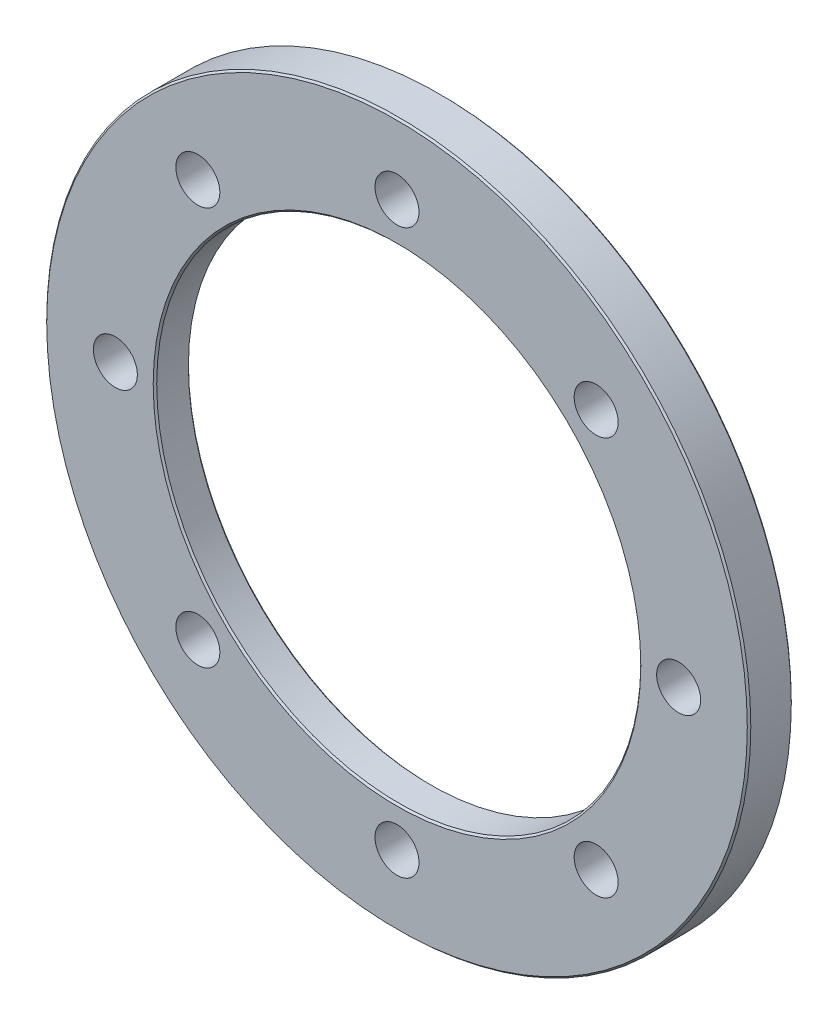
SolidWorks part; units mm, degrees
material "42CrMo"
ref_plane "Front Plane" through (0, 0, 0) normal (0, 0, 1) x (1, 0, 0)
ref_plane "Top Plane" through (0, 0, 0) normal (0, 1, 0) x (1, 0, 0)
ref_plane "Right Plane" through (0, 0, 0) normal (1, 0, 0) x (0, 0, -1)
sketch "Sketch1" plane through (0, 0, 0) normal (0, 0, 1) x (1, 0, 0)
  circle A0 centre (0, 0) radius 137.5
  circle A1 centre (0, 0) radius 200
  circle A2 centre (0, 0) radius 160 construction
  circle A3 centre (0, 160) radius 12.5
  circle A4 centre (113.1371, 113.1371) radius 12.5
  circle A5 centre (160, 0) radius 12.5
  circle A6 centre (113.1371, -113.1371) radius 12.5
  circle A7 centre (0, -160) radius 12.5
  circle A8 centre (-113.1371, -113.1371) radius 12.5
  circle A9 centre (-160, 0) radius 12.5
  circle A10 centre (-113.1371, 113.1371) radius 12.5
  point P23 (0, 0)
  dimension "D1" = 275
  dimension "D2" = 400
  dimension "D3" = 320
  dimension "D4" = 25
  dimension "D5" = 8
extrude "Boss-Extrude1" add sketch "Sketch1" along normal blind 25
chamfer "Chamfer1" distance 1 angle 45 4 edges at (137.5, 0, 0) (137.5, 0, 25) (200, 0, 0) (200, 0, 25)
sketch "Sketch2" plane through (0, 0, 0) normal (0, 0, 1) x (1, 0, 0)
  line L0 (0, 0) -> (0, 210.8893) construction
sketch "Sketch4" plane through (0, 0, 0) normal (0, 0, -1) x (-1, 0, 0)
  circle A0 centre (0, 0) radius 177.5
  dimension "D1" = 355
extrude "Cut-Extrude2" cut sketch "Sketch4" against normal blind 5
fillet "Fillet1" radius 2 1 edges at (-177.5, 0, 5)
chamfer "Chamfer2" distance 1 angle 45 2 edges at (-137.5, 0, 5) (-177.5, 0, 0)
